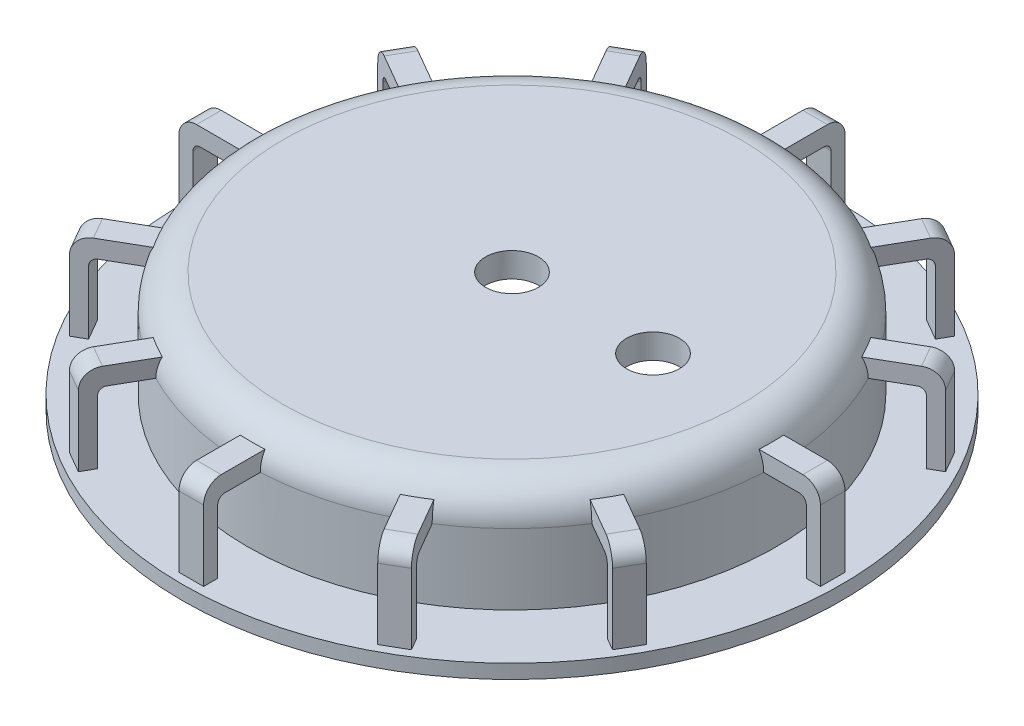
from build123d import *

# Parameters (mm, degrees)
SKETCH1_R                = 75
BOSS_EXTRUDE1_DEPTH      = 34
SKETCH3_R                = 93.5
BOSS_EXTRUDE2_DEPTH      = 4
FILLET1_R                = 10
SKETCH4_R                = 50
CUT_EXTRUDE1_DEPTH       = 27
SKETCH6_W                = 4
SKETCH6_H                = 7
BOSS_EXTRUDE3_DEPTH      = 25
BOSS_EXTRUDE4_REACH      = 208.103
SKETCH7_W                = 7
SKETCH7_H                = 5
FILLET2_R                = 5
FILLET3_R                = 2
CIRPATTERN2_COUNT        = 12
FILLET2_OF_CIRPATTERN2_R = 5
FILLET3_OF_CIRPATTERN2_R = 2
SKETCH8_R                = 7.5
CUT_EXTRUDE2_DEPTH       = 137.530216436


with BuildPart() as part:
    # Sketch1 → Boss-Extrude1 (new body)
    with BuildSketch(Plane(origin=(0, 0, 0), x_dir=(1, 0, 0), z_dir=(0, 1, 0))):
        with Locations(Location((0, 0, 0), (0, 0, 270))):
            Circle(SKETCH1_R)
    extrude(amount=BOSS_EXTRUDE1_DEPTH)

    # Sketch3 → Boss-Extrude2 (add)
    with BuildSketch(Plane(origin=(0, 0, 0), x_dir=(1, 0, 0), z_dir=(0, 1, 0))):
        with Locations(Location((0, 0, 0), (0, 0, 270))):
            Circle(SKETCH3_R)
    extrude(amount=BOSS_EXTRUDE2_DEPTH)

    # Fillet1
    fillet1_edges = [part.edges().sort_by_distance(p)[0] for p in [
        (0, 34, -75),
    ]]
    fillet(fillet1_edges, radius=FILLET1_R)

    # Sketch4 → Cut-Extrude1 (cut)
    with BuildSketch(Plane.XZ):
        with Locations(Location((0, 0, 0), (0, 0, 270))):
            Circle(SKETCH4_R)
    extrude(amount=-CUT_EXTRUDE1_DEPTH, mode=Mode.SUBTRACT)

    # Sketch6 → Boss-Extrude3 (add)
    with BuildSketch(Plane(origin=(0, 4, 0), x_dir=(1, 0, 0), z_dir=(0, 1, 0))):
        with Locations((89, 0)):
            Rectangle(SKETCH6_W, SKETCH6_H)
    boss_extrude3 = extrude(amount=BOSS_EXTRUDE3_DEPTH)

    # Sketch7 → Boss-Extrude4 (add, up to next)
    with BuildSketch(Plane.ZY.offset(-87), mode=Mode.PRIVATE) as boss_extrude4_sk1:
        with Locations((0, 26.5)):
            Rectangle(SKETCH7_W, SKETCH7_H)
    boss_extrude4_tool1 = extrude(boss_extrude4_sk1.sketch, amount=BOSS_EXTRUDE4_REACH, mode=Mode.PRIVATE) - part.part
    boss_extrude4 = boss_extrude4_tool1.solids().sort_by_distance((87, 26.5, 0))[0]
    add(boss_extrude4)

    # Fillet2
    fillet2_edges = [part.edges().sort_by_distance(p)[0] for p in [
        (91, 29, 0),
    ]]
    fillet(fillet2_edges, radius=FILLET2_R)

    # Fillet3
    fillet3_edges = [part.edges().sort_by_distance(p)[0] for p in [
        (87, 24, 0),
    ]]
    fillet(fillet3_edges, radius=FILLET3_R)

    # CirPattern2: Boss-Extrude3, Boss-Extrude4 ×12 about axis
    cirpattern2_axis = Axis((0, 0, 0), (0, 1, 0))
    add([boss_extrude3.rotate(cirpattern2_axis, i * 360 / CIRPATTERN2_COUNT) for i in range(1, CIRPATTERN2_COUNT)])
    add([boss_extrude4.rotate(cirpattern2_axis, i * 360 / CIRPATTERN2_COUNT) for i in range(1, CIRPATTERN2_COUNT)])

    # Fillet2 of CirPattern2
    fillet2_of_cirpattern2_edges = [part.edges().sort_by_distance(p)[0] for p in [
        (78.808311744, 29, -45.5),
        (45.5, 29, -78.808311744),
        (0, 29, -91),
        (-45.5, 29, -78.808311744),
        (-78.808311744, 29, -45.5),
        (-91, 29, 0),
        (-78.808311744, 29, 45.5),
        (-45.5, 29, 78.808311744),
        (0, 29, 91),
        (45.5, 29, 78.808311744),
        (78.808311744, 29, 45.5),
    ]]
    fillet(fillet2_of_cirpattern2_edges, radius=FILLET2_OF_CIRPATTERN2_R)

    # Fillet3 of CirPattern2
    fillet3_of_cirpattern2_edges = [part.edges().sort_by_distance(p)[0] for p in [
        (75.344210129, 24, -43.5),
        (43.5, 24, -75.344210129),
        (0, 24, -87),
        (-43.5, 24, -75.344210129),
        (-75.344210129, 24, -43.5),
        (-87, 24, 0),
        (-75.344210129, 24, 43.5),
        (-43.5, 24, 75.344210129),
        (0, 24, 87),
        (43.5, 24, 75.344210129),
        (75.344210129, 24, 43.5),
    ]]
    fillet(fillet3_of_cirpattern2_edges, radius=FILLET3_OF_CIRPATTERN2_R)

    # Sketch8 → Cut-Extrude2 (cut, through all)
    with BuildSketch(Plane(origin=(0, 34, 0), x_dir=(1, 0, 0), z_dir=(0, 1, 0))):
        with Locations(Location((0, 0, 0), (0, 0, 270))):
            Circle(SKETCH8_R)
        with Locations(Location((40, 0, 0), (0, 0, 90))):
            Circle(SKETCH8_R)
    extrude(amount=-CUT_EXTRUDE2_DEPTH, mode=Mode.SUBTRACT)


solid = part.part
